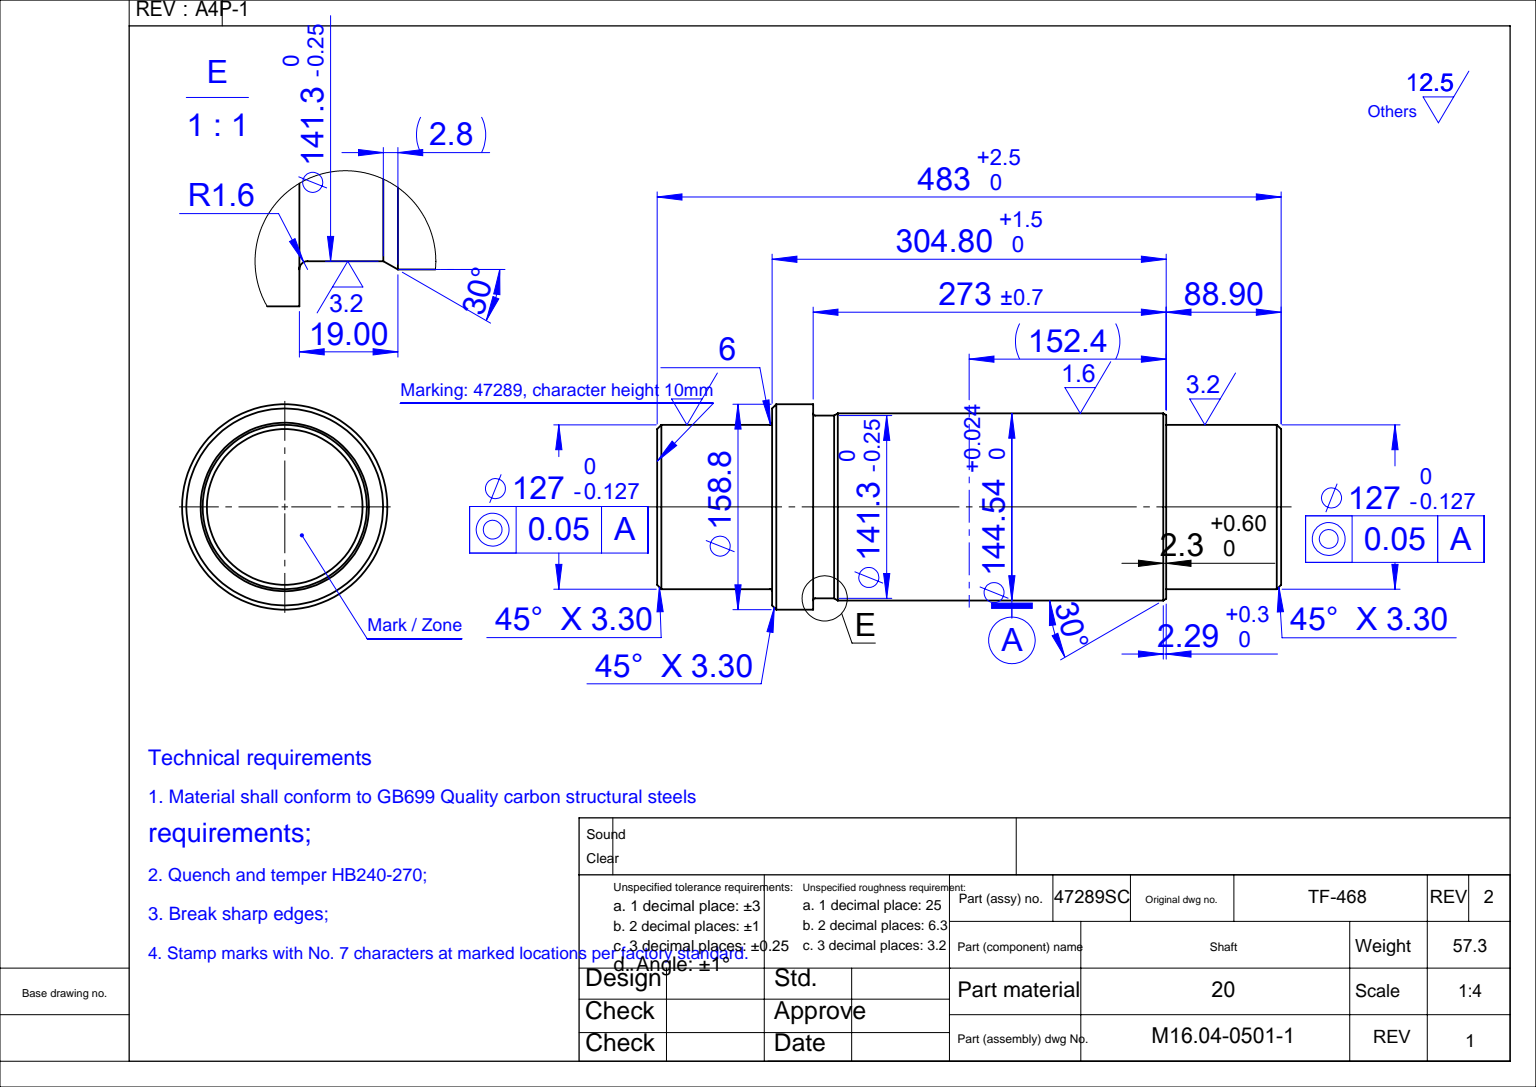
from build123d import *


with BuildPart() as part:
    # Sketch1 → Revolve1 (revolve)
    with BuildSketch(Plane(origin=(0, 0, 0), x_dir=(0, 0, -1), z_dir=(1, 0, 0)), mode=Mode.PRIVATE) as revolve1_sk:
        with BuildLine():
            Line((-237.998, 63.5), (-153.9875, 63.5))
            ThreePointArc((-153.9875, 63.5), (-152.864967985, 63.964967985), (-152.4, 65.0875))
            Line((-152.4, 65.0875), (-152.4, 76.073))
            Line((-152.4, 76.073), (-149.098, 79.375))
            Line((-149.098, 79.375), (-120.65, 79.375))
            Line((-120.65, 79.375), (-120.65, 72.2376))
            ThreePointArc((-120.65, 72.2376), (-120.185032015, 71.115067985), (-119.0625, 70.6501))
            Line((-119.0625, 70.6501), (-104.40462327, 70.6501))
            Line((-104.40462327, 70.6501), (-101.6, 72.26935))
            Line((-101.6, 72.26935), (150.114, 72.26935))
            Line((150.114, 72.26935), (152.4, 70.949527285))
            Line((152.4, 70.949527285), (152.4, 63.5))
            Line((152.4, 63.5), (237.998, 63.5))
            Line((237.998, 63.5), (241.3, 60.198))
            Line((241.3, 60.198), (241.3, 0))
            Line((241.3, 0), (-241.3, 0))
            Line((-241.3, 0), (-241.3, 60.198))
            Line((-241.3, 60.198), (-237.998, 63.5))
        make_face()
    revolve(revolve1_sk.sketch.rotate(Axis((0, 0, 264.578884175), (0, 0, -1)), 90), axis=Axis((0, 0, 264.578884175), (0, 0, -1)))


solid = part.part
